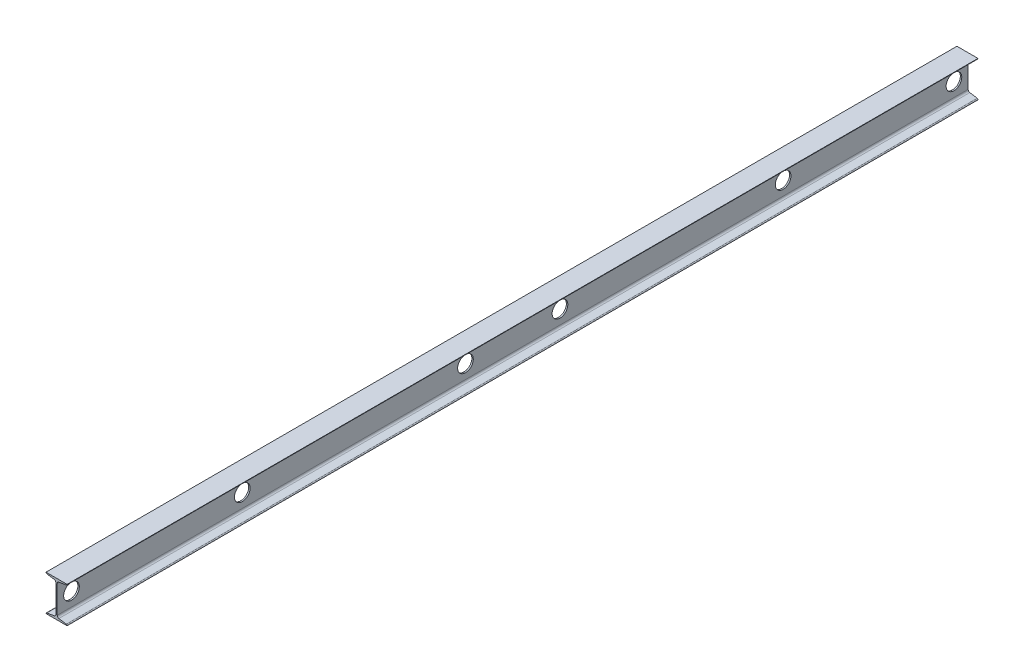
SolidWorks part; units mm, degrees
material "普通碳钢"
ref_plane "Front Plane" through (0, 0, 0) normal (0, 0, 1) x (1, 0, 0)
ref_plane "Top Plane" through (0, 0, 0) normal (0, 1, 0) x (1, 0, 0)
ref_plane "Right Plane" through (0, 0, 0) normal (1, 0, 0) x (0, 0, -1)
sketch "Sketch1" plane through (0, 0, 0) normal (0, 0, 1) x (1, 0, 0)
  line L0 (-2.5, 48.4) -> (-2.5, -48.4)
  line L1 (-34.0695, -59.5466) -> (-8.3609, -55.3067)
  line L2 (-37, 63) -> (37, 63)
  line L3 (-37, -63) -> (37, -63)
  line L4 (-19.7759, 48.4) -> (29.2827, 48.4) construction
  line L5 (-34.0695, 59.5466) -> (-8.3609, 55.3067)
  line L6 (-28.6128, 0) -> (37, 0) construction
  line L7 (0, 0) -> (0, 91.7442) construction
  line L8 (28.6128, 0) -> (-37, 0) construction
  line L9 (19.7759, 48.4) -> (-29.2827, 48.4) construction
  line L10 (34.0695, 59.5466) -> (8.3609, 55.3067)
  line L11 (34.0695, -59.5466) -> (8.3609, -55.3067)
  line L12 (2.5, 48.4) -> (2.5, -48.4)
  arc A0 (-37, 63) -> (-34.0695, 59.5466) centre (-33.5, 63) ccw
  arc A1 (-2.5, 48.4) -> (-8.3609, 55.3067) centre (-9.5, 48.4) ccw
  arc A2 (-2.5, -48.4) -> (-8.3609, -55.3067) centre (-9.5, -48.4) cw
  arc A3 (-37, -63) -> (-34.0695, -59.5466) centre (-33.5, -63) cw
  arc A4 (37, -63) -> (34.0695, -59.5466) centre (33.5, -63) ccw
  arc A5 (2.5, -48.4) -> (8.3609, -55.3067) centre (9.5, -48.4) ccw
  arc A6 (2.5, 48.4) -> (8.3609, 55.3067) centre (9.5, 48.4) cw
  arc A7 (37, 63) -> (34.0695, 59.5466) centre (33.5, 63) cw
  point P3 (-2.5, 0)
  point P6 (2.5, 0)
  point P19 (0, 63)
  point P38 (0, -63)
  dimension "D7" = 7
  dimension "D9" = 14
  dimension "D1" = 2.5
  dimension "D2" = 63
  dimension "D6" = 37
  dimension "D8" = 48.4
extrude "Boss-Extrude1" add sketch "Sketch1" along normal blind 3200
sketch "Sketch2" plane through (2.5, 0, 0) normal (1, 0, 0) x (0, 0, -1)
  line L0 (0, 0) -> (-3402.5904, 0) construction
  line L1 (-50, 347.1871) -> (-50, -268.0287) construction
  line L2 (-650, 419.8427) -> (-650, -318.6847) construction
  line L3 (-1434, 375.9324) -> (-1434, -318.6847) construction
  line L4 (-1766, 419.8427) -> (-1766, -509.0656) construction
  line L5 (-2550, 465.0096) -> (-2550, -452.6789) construction
  line L6 (-2550, 419.8427) -> (-2550, -509.0656) construction
  line L7 (-3150, 504.1124) -> (-3150, -646.041) construction
  circle A0 centre (-50, 0) radius 27.5
  circle A1 centre (-650, 0) radius 27.5
  circle A2 centre (-1434, 0) radius 27.5
  circle A3 centre (-1766, 0) radius 27.5
  circle A4 centre (-2550, 0) radius 27.5
  circle A5 centre (-3150, 0) radius 27.5
  dimension "D7" = 55
  dimension "D1" = 50
  dimension "D2" = 600
  dimension "D3" = 784
  dimension "D4" = 332
  dimension "D5" = 784
  dimension "D6" = 600
extrude "Cut-Extrude1" cut sketch "Sketch2" against normal up to next
